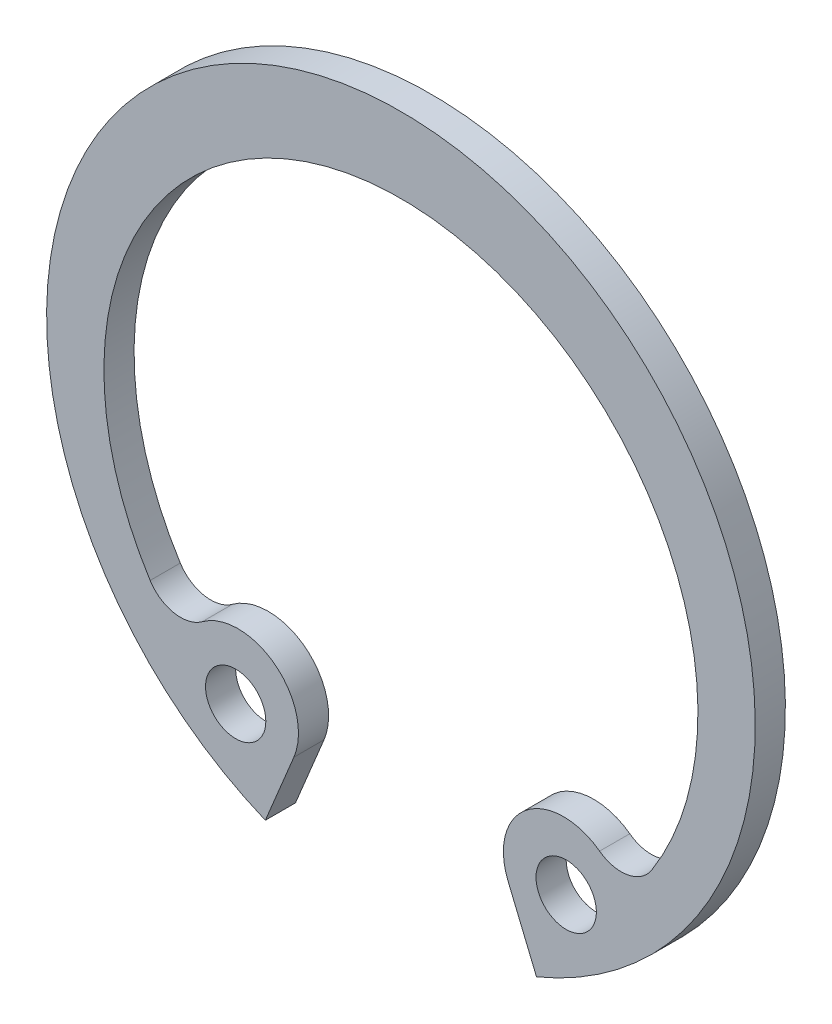
from build123d import *

# Parameters (mm, degrees)
BASE_EXTRUDE_DEPTH      = 0.5
BASE_EXTRUDE_DEPTH_BACK = 0.5
SKETCH1_R               = 1


with BuildPart() as part:
    # Sketch1 → Base-Extrude (new, two sides: drawn at the far end of the back side and taken through both)
    with BuildSketch(Plane.XY.offset(-BASE_EXTRUDE_DEPTH_BACK)):
        with BuildLine():
            Line((-3.550099977, -8.570699513), (-4.49653033, -10.855584507))
            ThreePointArc((-4.49653033, -10.855584507), (0, 11.75), (4.49653033, -10.855584507))
            Line((4.49653033, -10.855584507), (3.550099977, -8.570699513))
            ThreePointArc((3.550099977, -8.570699513), (4.167236093, -6.228764491), (6.588932053, -6.198676157))
            ThreePointArc((6.588932053, -6.198676157), (7.52278189, -6.414491024), (8.316788695, -5.877643962))
            ThreePointArc((8.316788695, -5.877643962), (0, 9.25), (-8.316788695, -5.877643962))
            ThreePointArc((-8.316788695, -5.877643962), (-7.52278189, -6.414491024), (-6.588932053, -6.198676157))
            ThreePointArc((-6.588932053, -6.198676157), (-4.167236093, -6.228764491), (-3.550099977, -8.570699513))
        make_face()
        with Locations((-5.480027646, -8.003705205)):
            Circle(SKETCH1_R, mode=Mode.SUBTRACT)
        with Locations(Location((5.480027646, -8.003705205, 0), (0, 0, 180))):
            Circle(SKETCH1_R, mode=Mode.SUBTRACT)
    extrude(amount=BASE_EXTRUDE_DEPTH + BASE_EXTRUDE_DEPTH_BACK)


solid = part.part
